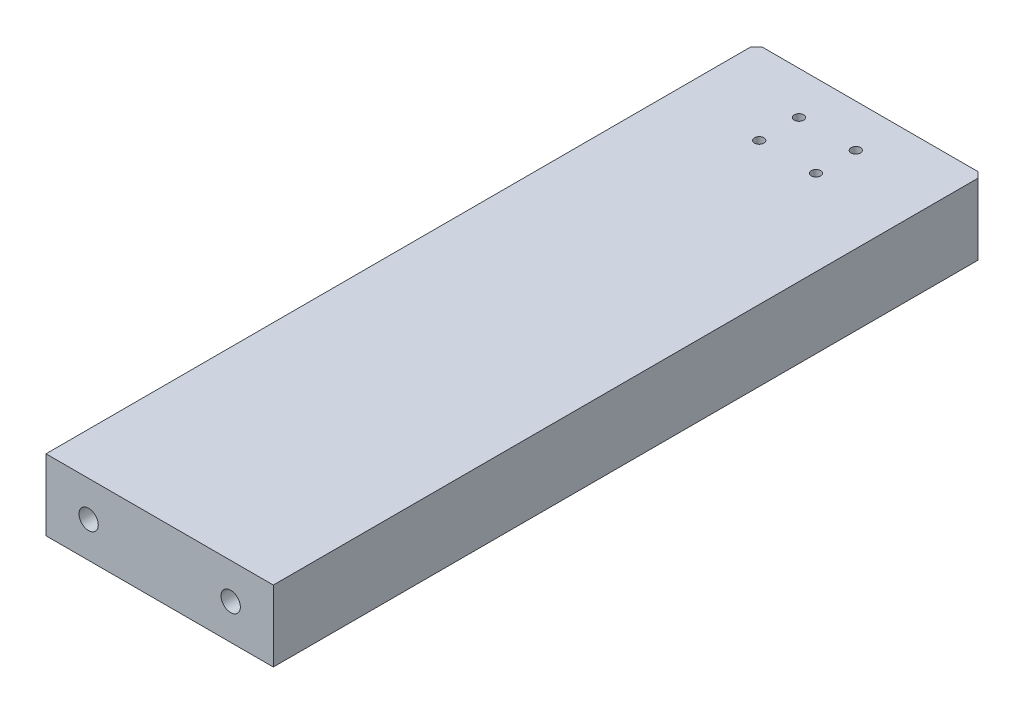
SolidWorks part; units mm, degrees
material "Q235"
ref_plane "Front Plane" through (0, 0, 0) normal (0, 0, 1) x (1, 0, 0)
ref_plane "Top Plane" through (0, 0, 0) normal (0, 1, 0) x (1, 0, 0)
ref_plane "Right Plane" through (0, 0, 0) normal (1, 0, 0) x (0, 0, -1)
sketch "Sketch1" plane through (0, 0, 0) normal (0, 1, 0) x (1, 0, 0)
  line L0 (-75, 0) -> (75, 0)
  line L1 (75, 0) -> (75, 12)
  line L2 (75, 12) -> (40, 12)
  line L3 (40, 12) -> (40, 250)
  line L4 (40, 250) -> (-40, 250)
  line L5 (-40, 250) -> (-40, 12)
  line L6 (-40, 12) -> (-75, 12)
  line L7 (-75, 12) -> (-75, 0)
  line L8 (0, 250) -> (0, 0) construction
  dimension "D1" = 150
  dimension "D2" = 250
  dimension "D3" = 12
  dimension "D4" = 80
extrude "Boss-Extrude1" add sketch "Sketch1" along normal mid plane 25
chamfer "Chamfer1" distance 2 angle 45 4 edges at (75, 0, -12) (40, 0, -250) (-75, 0, -12) (-40, 0, -250)
hole_wizard "Hole1" positions "Sketch2" profile "Sketch3" legacy end condition through all
sketch "Sketch2" plane through (0, 0, 0) normal (0, 0, 1) x (1, 0, 0)
  line L0 (-75, 0) -> (75, 0) construction
  line L1 (-75, 12.5) -> (-75, -12.5) construction
  line L2 (75, 12.5) -> (75, -12.5) construction
  point P0 (-60, 0)
  point P2 (60, 0)
  dimension "D1" = 120
  dimension "D2" = 15
sketch "Sketch3" plane through (-60, 0, 0) normal (1, 0, 0) x (0, -1, 0)
  line L0 (0, 0) -> (0, 250)
  line L1 (0, 250) -> (4.5, 250)
  line L2 (4.5, 250) -> (4.5, 0)
  line L3 (4.5, 0) -> (0, 0)
  line L4 (0, 110) -> (0, -10) construction
  dimension "直径" = 9
  dimension "深度" = 250
sketch "Sketch4" plane through (0, -12.5, 0) normal (0, -1, 0) x (-1, 0, 0)
  line L0 (0, 250) -> (0, 0) construction
  line L1 (-38, 250) -> (38, 250) construction
  line L2 (0, 80) -> (0, 250) construction
  line L3 (-13.5, 80) -> (-13.5, 250)
  line L4 (13.5, 80) -> (13.5, 250)
  arc A0 (-13.5, 80) -> (13.5, 80) centre (0, 80) ccw
  arc A1 (13.5, 250) -> (-13.5, 250) centre (0, 250) ccw
  point P6 (0, 165)
  dimension "D2" = 13.5
  dimension "D1" = 170
extrude "Cut-Extrude1" cut sketch "Sketch4" against normal blind 15
hole_wizard "M8 Tapped Hole1" positions "Sketch5" profile "Sketch6" tap size "M8" standard "GB"
sketch "Sketch5" plane through (35, 0, 0) normal (1, 0, 0) x (0, 0, -1)
  line L0 (250, 0) -> (0, 0) construction
  line L1 (250, 12.5) -> (250, -12.5) construction
  line L2 (0, 12.5) -> (0, -12.5) construction
  point P11 (225, 0)
  point P13 (50, 0)
  point P15 (30, 0)
  dimension "D1" = 30
  dimension "D2" = 20
  dimension "D3" = 195
sketch "Sketch6" plane through (35, 0, -30) normal (0, 1, 0) x (0, 0, -1)
  line L0 (0, 0) -> (0, 21.7929)
  line L1 (0, 21.7929) -> (3.4, 19.75)
  line L2 (3.4, 19.75) -> (3.4, 0.625)
  line L3 (3.4, 0.625) -> (4.025, 0)
  line L5 (4.025, 0) -> (0, 0)
  line L6 (-3.4, 0.625) -> (-4.025, 0) construction
  line L10 (0, 21.7929) -> (-3.4, 19.75) construction
  line L11 (0, -6.35) -> (0, 107.95) construction
  dimension "螺纹孔钻头直径" = 6.8
  dimension "螺纹孔钻头深度" = 19.75
  dimension "近端锥形沉头孔直径" = 8.05
  dimension "近端锥形沉头孔角度" = 90
  dimension "导头角度" = 118
cosmetic thread "Hole thread 1" [suppressed] parameters "D1"=16, "D2"=8
cosmetic thread "Hole thread 2" [suppressed] parameters "D1"=16, "D2"=8
cosmetic thread "Hole thread 3" [suppressed] parameters "D1"=16, "D2"=8
mirror "Mirror1" about plane through (0, 0, 0) normal (1, 0, 0)
cosmetic thread "Hole thread 4" [suppressed] parameters "D1"=16, "D2"=8
cosmetic thread "Hole thread 5" [suppressed] parameters "D1"=16, "D2"=8
cosmetic thread "Hole thread 6" [suppressed] parameters "D1"=16, "D2"=8
hole_wizard "M5 Tapped Hole1" positions "Sketch7" profile "Sketch8" tap size "M5" standard "GB"
sketch "Sketch7" plane through (0, 12.5, 0) normal (0, 1, 0) x (1, 0, 0)
  line L0 (-13.5, 240) -> (-13.5, 0) construction
  line L1 (25, 240) -> (-25, 240) construction
  line L2 (-65, 0) -> (65, 0) construction
  point P10 (-13.5, 232.5)
  point P12 (-13.5, 209.5)
  point P14 (-13.5, 186.5)
  dimension "D1" = 23
  dimension "D2" = 23
  dimension "D3" = 7.5
  dimension "D4" = 13.5
sketch "Sketch8" plane through (-13.5, 12.5, -186.5) normal (1, 0, 0) x (0, 0, 1)
  line L0 (0, 0) -> (0, 16.2618)
  line L1 (0, 16.2618) -> (2.1, 15)
  line L2 (2.1, 15) -> (2.1, 0.425)
  line L3 (2.1, 0.425) -> (2.525, 0)
  line L5 (2.525, 0) -> (0, 0)
  line L6 (-2.1, 0.425) -> (-2.525, 0) construction
  line L10 (0, 16.2618) -> (-2.1, 15) construction
  line L11 (0, -6.35) -> (0, 107.95) construction
  dimension "螺纹孔钻头直径" = 4.2
  dimension "螺纹孔钻头深度" = 15
  dimension "近端锥形沉头孔直径" = 5.05
  dimension "近端锥形沉头孔角度" = 90
  dimension "导头角度" = 118
cosmetic thread "Hole thread 7" [suppressed] parameters "D1"=12, "D2"=5
cosmetic thread "Hole thread 8" [suppressed] parameters "D1"=12, "D2"=5
cosmetic thread "Hole thread 9" [suppressed] parameters "D1"=12, "D2"=5
mirror "Mirror2" about plane through (0, 0, 0) normal (1, 0, 0)
cosmetic thread "Hole thread 10" [suppressed] parameters "D1"=12, "D2"=5
cosmetic thread "Hole thread 11" [suppressed] parameters "D1"=12, "D2"=5
cosmetic thread "Hole thread 12" [suppressed] parameters "D1"=12, "D2"=5
hole_wizard "M4 Tapped Hole1" positions "Sketch9" profile "Sketch10" tap size "M4" standard "GB" end condition through all
sketch "Sketch9" plane through (0, 12.5, 0) normal (0, 1, 0) x (1, 0, 0)
  line L0 (0, 250) -> (0, 237.7487) construction
  line L1 (38, 250) -> (-38, 250) construction
  point P0 (-10, 235)
  point P2 (-10, 221)
  point P12 (10, 221)
  point P13 (10, 235)
  dimension "D1" = 20
  dimension "D2" = 14
  dimension "D3" = 15
sketch "Sketch10" plane through (-10, 12.5, -235) normal (1, 0, 0) x (0, 0, 1)
  line L0 (0, 0) -> (0, 25)
  line L1 (0, 25) -> (1.65, 25)
  line L2 (1.65, 25) -> (1.65, 0)
  line L5 (1.65, 0) -> (0, 0)
  line L11 (0, -6.35) -> (0, 107.95) construction
  dimension "通孔螺纹孔钻头直径" = 3.3
  dimension "通孔螺纹孔钻头深度" = 25
cosmetic thread "Hole thread 13" parameters "D2"=4
cosmetic thread "Hole thread 14" parameters "D2"=4
cosmetic thread "Hole thread 15" parameters "D2"=4
cosmetic thread "Hole thread 16" parameters "D2"=4
sketch "Sketch11" plane through (0, 0, -12) normal (0, 0, -1) x (-1, 0, 0)
  line L1 (-75, 12.5) -> (-40, 12.5)
  line L2 (-75, 12.5) -> (-75, -12.5)
  line L3 (-75, -12.5) -> (-40, -12.5)
  line L4 (-40, 12.5) -> (-40, -12.5)
  line L5 (75, 12.5) -> (40, 12.5)
  line L6 (75, 12.5) -> (75, -12.5)
  line L7 (75, -12.5) -> (40, -12.5)
  line L8 (40, 12.5) -> (40, -12.5)
extrude "Cut-Extrude2" cut sketch "Sketch11" against normal through all
hole_wizard "M8 Tapped Hole2" positions "Sketch12" profile "Sketch13" tap size "M8" standard "GB"
sketch "Sketch12" plane through (0, 0, 0) normal (0, 0, 1) x (1, 0, 0)
  line L0 (0, 12.5) -> (0, -12.5) construction
  line L1 (-40, 12.5) -> (40, 12.5) construction
  line L2 (-40, -12.5) -> (40, -12.5) construction
  line L4 (-40, 0) -> (-25, 0) construction
  line L5 (-40, 12.5) -> (-40, -12.5) construction
  point P0 (-25, 0)
  point P2 (25, 0)
  dimension "D1" = 50
cosmetic thread "Hole thread 17" parameters "D1"=16, "D2"=8
cosmetic thread "Hole thread 18" parameters "D1"=16, "D2"=8
sketch "Sketch13" plane through (-25, 0, 0) normal (1, 0, 0) x (0, -1, 0)
  line L0 (0, 0) -> (0, 21.7929)
  line L1 (0, 21.7929) -> (3.4, 19.75)
  line L2 (3.4, 19.75) -> (3.4, 0)
  line L5 (3.4, 0) -> (0, 0)
  line L10 (0, 21.7929) -> (-3.4, 19.75) construction
  line L11 (0, -6.35) -> (0, 107.95) construction
  dimension "螺纹孔钻头直径" = 6.8
  dimension "螺纹孔钻头深度" = 19.75
  dimension "导头角度" = 118
